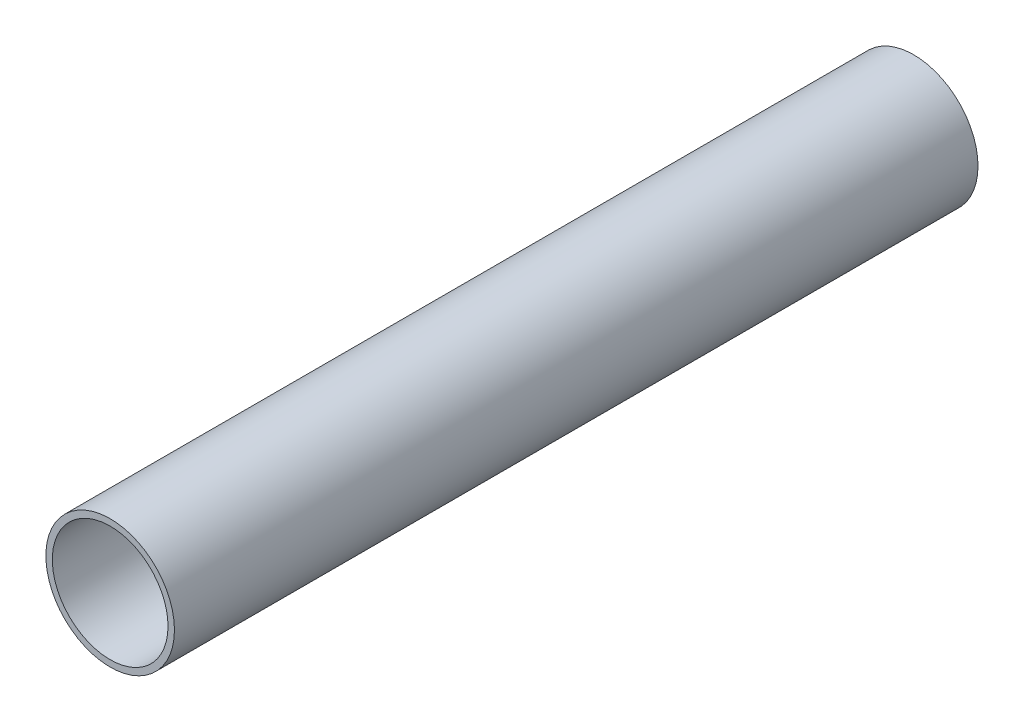
from build123d import *

# Parameters (mm, degrees)
SKETCH_1_R      = 20
SKETCH_1_R_2    = 18
EXTRUDE_1_DEPTH = 250


with BuildPart() as part:
    # 草图1 → 凸台-拉伸1 (new body)
    with BuildSketch(Plane.XY):
        Circle(SKETCH_1_R)
        Circle(SKETCH_1_R_2, mode=Mode.SUBTRACT)
    extrude(amount=EXTRUDE_1_DEPTH)


solid = part.part
